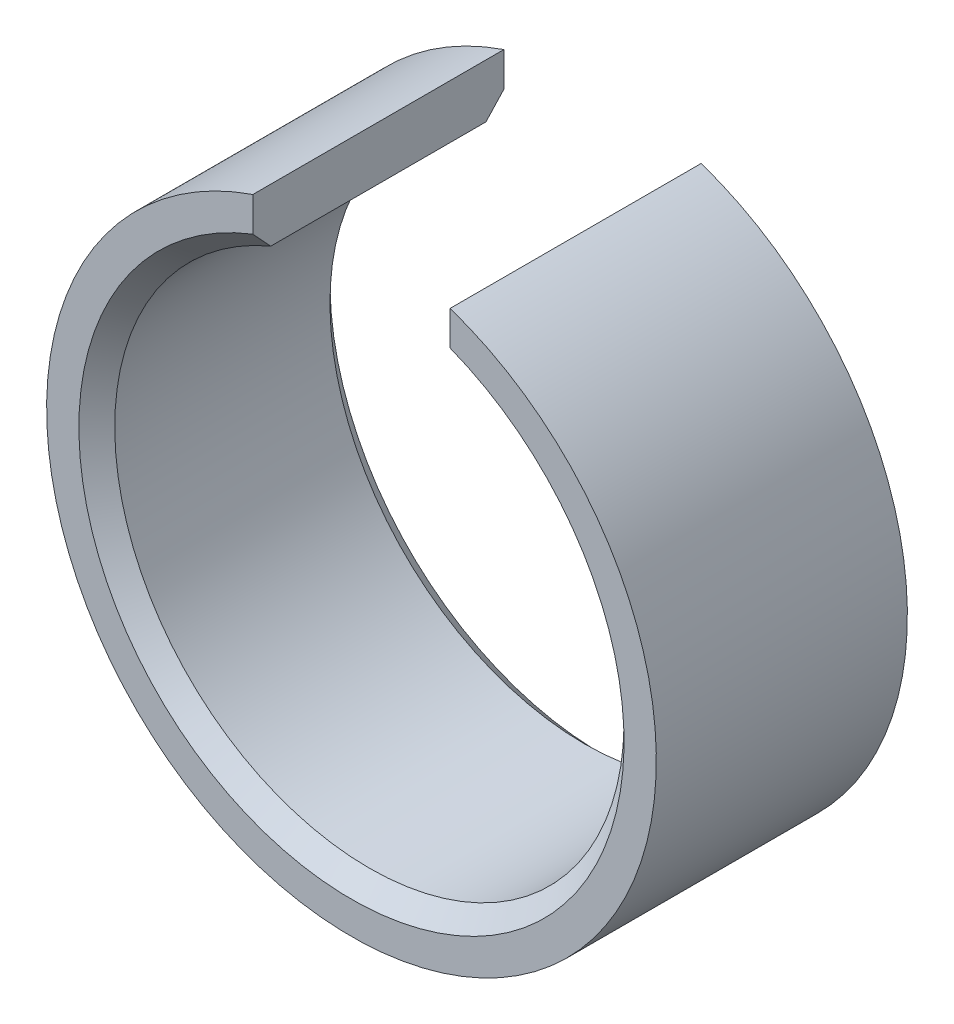
SolidWorks part; units mm, degrees
material "6061-T6 (GB)"
ref_plane "Front Plane" through (0, 0, 0) normal (0, 0, 1) x (1, 0, 0)
ref_plane "Top Plane" through (0, 0, 0) normal (0, 1, 0) x (1, 0, 0)
ref_plane "Right Plane" through (0, 0, 0) normal (1, 0, 0) x (0, 0, -1)
sketch "Sketch1" plane through (0, 0, 0) normal (0, 0, 1) x (1, 0, 0)
  circle A0 centre (0, 0) radius 7.1
  circle A1 centre (0, 0) radius 8.5
  dimension "D1" = 14.2
  dimension "D2" = 17
extrude "Boss-Extrude1" add sketch "Sketch1" along normal blind 7
sketch "Sketch2" plane through (0, 0, 7) normal (0, 0, 1) x (1, 0, 0)
  line L0 (0, 0) -> (0, 7.1) construction
  line L1 (2.75, 0) -> (-2.75, 0)
  line L2 (2.75, 0) -> (2.75, 15)
  line L3 (2.75, 15) -> (-2.75, 15)
  line L4 (-2.75, 0) -> (-2.75, 15)
  line L5 (2.75, 0) -> (-2.75, 15) construction
  line L6 (2.75, 15) -> (-2.75, 0) construction
  circle A0 centre (0, 0) radius 7.1 construction
  point P0 (0, 7.5)
  dimension "D1" = 5.5
  dimension "D2" = 15
extrude "Cut-Extrude1" cut sketch "Sketch2" against normal through all
chamfer "Chamfer1" distance 0.5 angle 45 2 edges at (0, -7.1, 0) (0, -7.1, 7)
